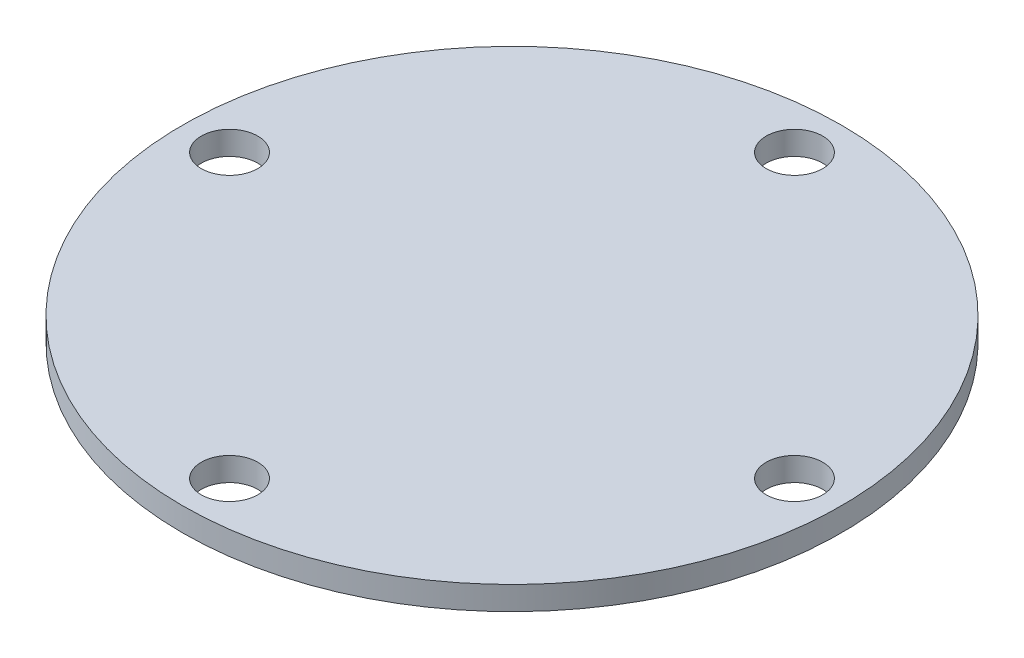
from build123d import *

# Parameters (mm, degrees)
SKETCH_1_R          = 70
EXTRUDE_1_DEPTH     = 5
SKETCH_3_R          = 6
CUT_EXTRUDE_1_DEPTH = 100.121138008


with BuildPart() as part:
    # 草图1 → 凸台-拉伸1 (new body)
    with BuildSketch(Plane(origin=(0, 0, 0), x_dir=(1, 0, 0), z_dir=(0, 1, 0))):
        with Locations(Location((0, 0, 0), (0, 0, 270))):
            Circle(SKETCH_1_R)
    extrude(amount=EXTRUDE_1_DEPTH)

    # 草图3 → 切除-拉伸1 (cut, through all)
    with BuildSketch(Plane(origin=(0, 5, 0), x_dir=(1, 0, 0), z_dir=(0, 1, 0))):
        with Locations(Location((0, 60, 0), (0, 0, 270))):
            Circle(SKETCH_3_R)
        with Locations(Location((60, 0, 0), (0, 0, 270))):
            Circle(SKETCH_3_R)
        with Locations(Location((0, -60, 0), (0, 0, 270))):
            Circle(SKETCH_3_R)
        with Locations(Location((-60, 0, 0), (0, 0, 270))):
            Circle(SKETCH_3_R)
    extrude(amount=-CUT_EXTRUDE_1_DEPTH, mode=Mode.SUBTRACT)


solid = part.part
